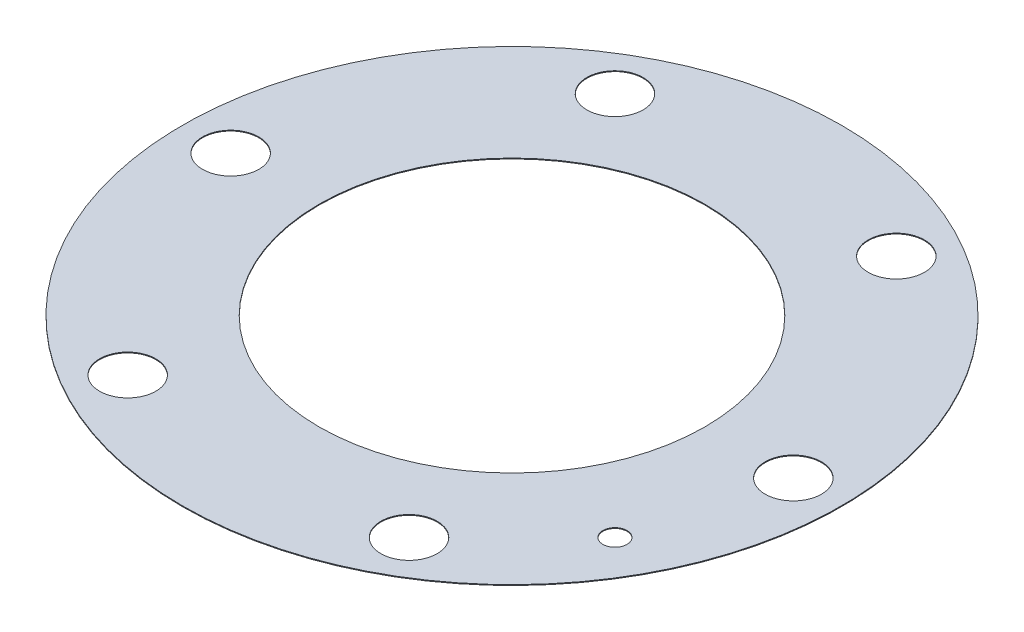
from build123d import *

# Parameters (mm, degrees)
SKETCH1_R           = 41
SKETCH1_R_2         = 24
SKETCH1_R_3         = 3.5
SKETCH1_R_4         = 1.5
BOSS_EXTRUDE1_DEPTH = 0.1


with BuildPart() as part:
    # Sketch1 → Boss-Extrude1 (new body)
    with BuildSketch(Plane(origin=(0, 0, 0), x_dir=(1, 0, 0), z_dir=(0, 1, 0))):
        with Locations(Location((0, 0, 0), (0, 0, 270))):
            Circle(SKETCH1_R)
        with Locations(Location((0, 0, 0), (0, 0, 270))):
            Circle(SKETCH1_R_2, mode=Mode.SUBTRACT)
        with Locations(Location((35, 0, 0), (0, 0, 270))):
            Circle(SKETCH1_R_3, mode=Mode.SUBTRACT)
        with Locations(Location((17.5, -30.310889132, 0), (0, 0, 270))):
            Circle(SKETCH1_R_3, mode=Mode.SUBTRACT)
        with Locations(Location((-17.5, -30.310889132, 0), (0, 0, 270))):
            Circle(SKETCH1_R_3, mode=Mode.SUBTRACT)
        with Locations(Location((-35, 0, 0), (0, 0, 270))):
            Circle(SKETCH1_R_3, mode=Mode.SUBTRACT)
        with Locations(Location((-17.5, 30.310889132, 0), (0, 0, 270))):
            Circle(SKETCH1_R_3, mode=Mode.SUBTRACT)
        with Locations(Location((17.5, 30.310889132, 0), (0, 0, 270))):
            Circle(SKETCH1_R_3, mode=Mode.SUBTRACT)
        with Locations(Location((30.310889132, -17.5, 0), (0, 0, 270))):
            Circle(SKETCH1_R_4, mode=Mode.SUBTRACT)
    extrude(amount=BOSS_EXTRUDE1_DEPTH)


solid = part.part
